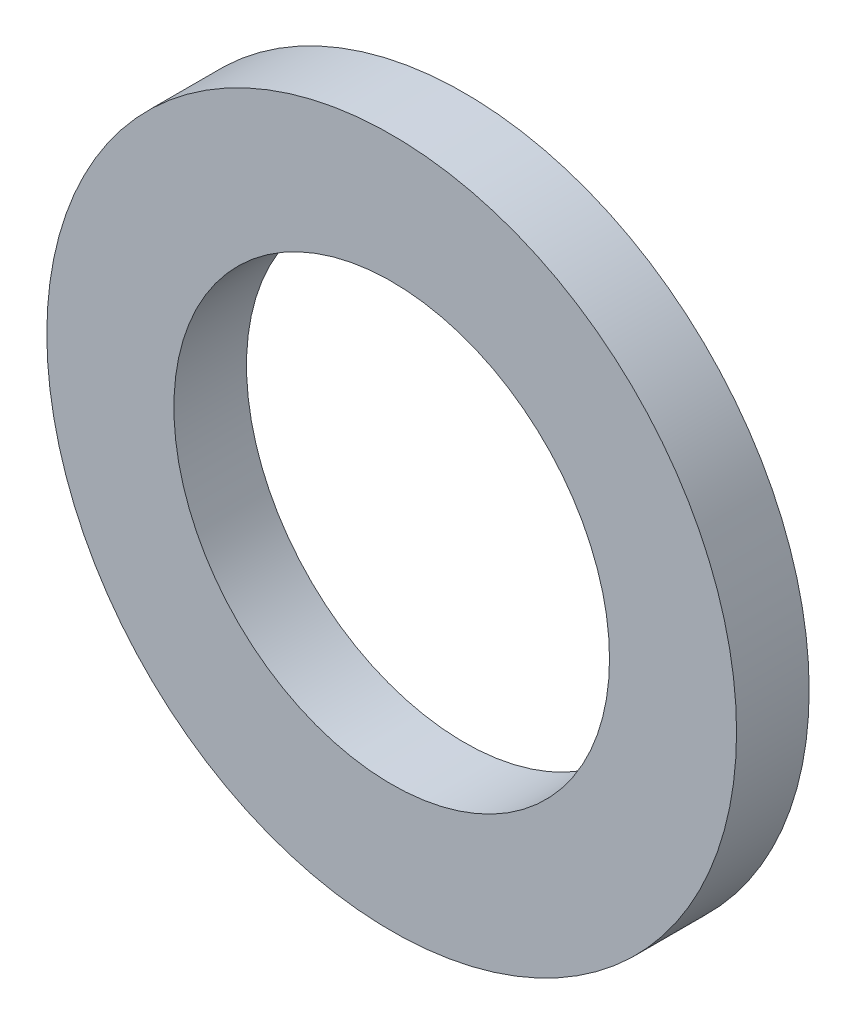
SolidWorks part; units mm, degrees
material "Aluminum bronze"
ref_plane "Front Plane" through (0, 0, 0) normal (0, 0, 1) x (1, 0, 0)
ref_plane "Top Plane" through (0, 0, 0) normal (0, 1, 0) x (1, 0, 0)
ref_plane "Right Plane" through (0, 0, 0) normal (1, 0, 0) x (0, 0, -1)
sketch "Sketch1" plane through (0, 0, 0) normal (0, 0, 1) x (1, 0, 0)
  circle A0 centre (0, 0) radius 24
  circle A1 centre (0, 0) radius 38
  dimension "D1" = 76
  dimension "D2" = 48
extrude "Boss-Extrude1" add sketch "Sketch1" along normal blind 8
